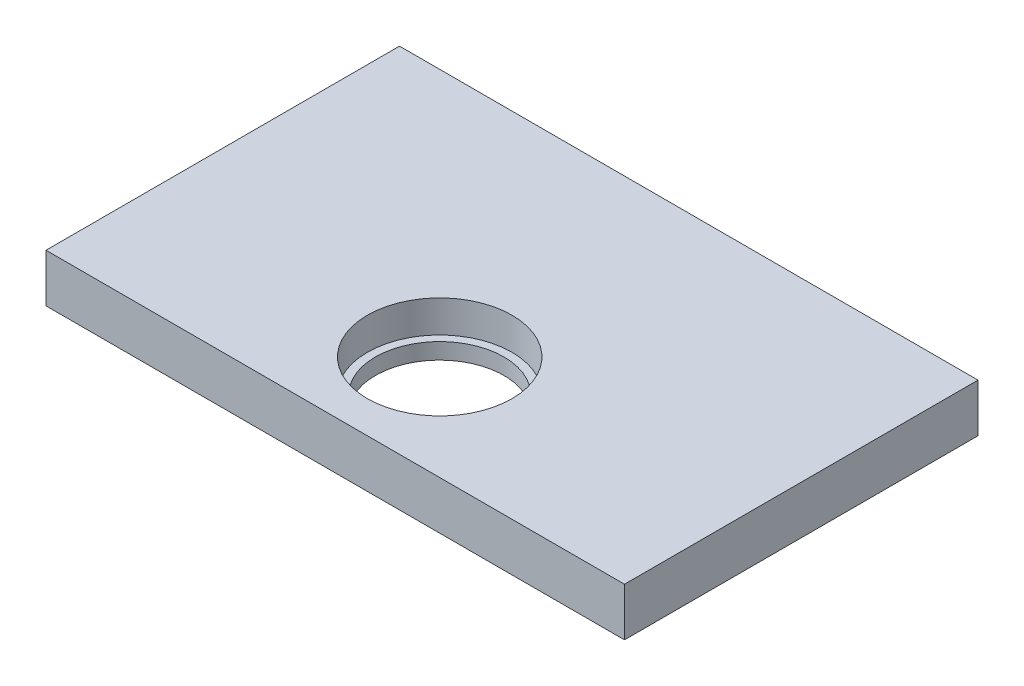
from build123d import *

# Parameters (mm, degrees)
SKETCH_1_W          = 360
SKETCH_1_H          = 220
EXTRUDE_1_DEPTH     = 30
SKETCH_2_R          = 40
CUT_EXTRUDE_1_DEPTH = 214.072757527
SKETCH_3_R          = 45
CUT_EXTRUDE_2_DEPTH = 20


with BuildPart() as part:
    # 草图1 → 凸台-拉伸1 (new body)
    with BuildSketch(Plane(origin=(0, 0, 0), x_dir=(1, 0, 0), z_dir=(0, 1, 0))):
        Rectangle(SKETCH_1_W, SKETCH_1_H)
    extrude(amount=EXTRUDE_1_DEPTH)

    # 草图2 → 切除-拉伸1 (cut, through all)
    with BuildSketch(Plane(origin=(0, 30, 0), x_dir=(1, 0, 0), z_dir=(0, 1, 0))):
        with Locations(Location((0, -45, 0), (0, 0, 270))):
            Circle(SKETCH_2_R)
    extrude(amount=-CUT_EXTRUDE_1_DEPTH, mode=Mode.SUBTRACT)

    # 草图3 → 切除-拉伸2 (cut)
    with BuildSketch(Plane.XZ.offset(-30)):
        with Locations(Location((0, 45, 0), (0, 0, 270))):
            Circle(SKETCH_3_R)
    extrude(amount=CUT_EXTRUDE_2_DEPTH, mode=Mode.SUBTRACT)


solid = part.part
